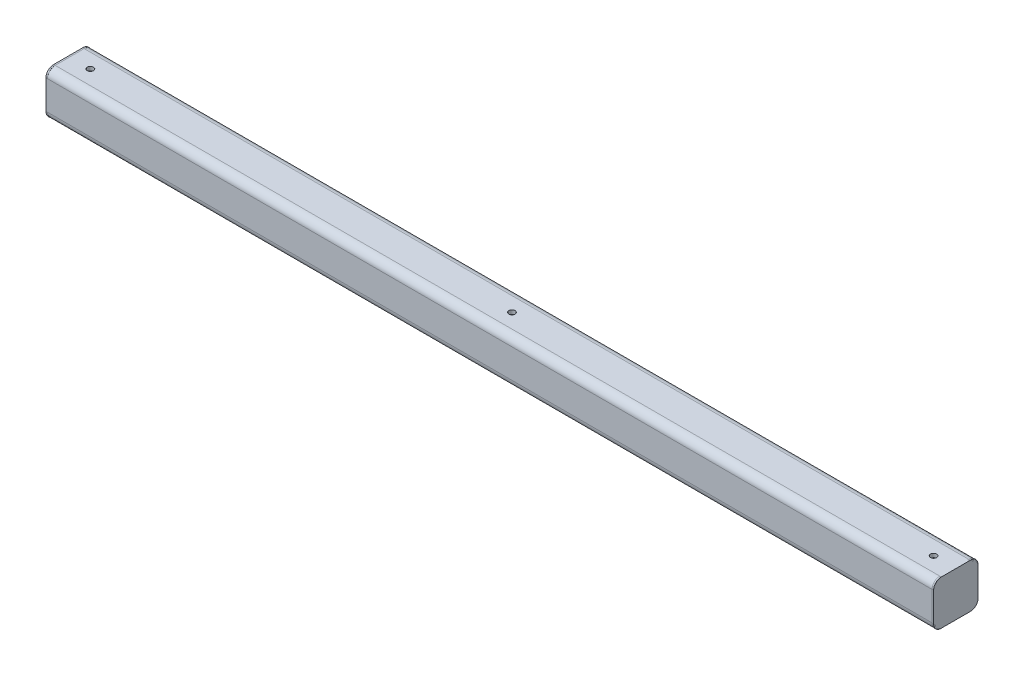
SolidWorks part; units mm, degrees
ref_plane "前视基准面" through (0, 0, 0) normal (0, 0, 1) x (1, 0, 0)
ref_plane "上视基准面" through (0, 0, 0) normal (0, 1, 0) x (1, 0, 0)
ref_plane "右视基准面" through (0, 0, 0) normal (1, 0, 0) x (0, 0, -1)
sketch3d "3D草图1"
  line L0 (0, 0, 0) -> (600, 0, 0)
  dimension "D1" = 600
other "结构构件1"
ref_plane "基准面1" through (0, 0, 0) normal (1, 0, 0) x (0, 0, -1)
sketch "Sketch1" plane through (0, 0, 0) normal (1, 0, 0) x (0, 0, -1)
  line L0 (-9.8, -12.4) -> (9.8, -12.4)
  line L1 (-12.4, -9.8) -> (-12.4, 9.8)
  line L2 (9.8, 12.4) -> (-9.8, 12.4)
  line L3 (12.4, 9.8) -> (12.4, -9.8)
  line L4 (-9.8, -15) -> (9.8, -15)
  line L5 (-15, -9.8) -> (-15, 9.8)
  line L6 (9.8, 15) -> (-9.8, 15)
  line L7 (15, 9.8) -> (15, -9.8)
  arc A0 (15, 9.8) -> (9.8, 15) centre (9.8, 9.8) ccw
  arc A1 (9.8, -15) -> (15, -9.8) centre (9.8, -9.8) ccw
  arc A2 (-15, -9.8) -> (-9.8, -15) centre (-9.8, -9.8) ccw
  arc A3 (-9.8, 15) -> (-15, 9.8) centre (-9.8, 9.8) ccw
  arc A4 (-9.8, 12.4) -> (-12.4, 9.8) centre (-9.8, 9.8) ccw
  arc A5 (12.4, 9.8) -> (9.8, 12.4) centre (9.8, 9.8) ccw
  arc A6 (9.8, -12.4) -> (12.4, -9.8) centre (9.8, -9.8) ccw
  arc A7 (-12.4, -9.8) -> (-9.8, -12.4) centre (-9.8, -9.8) ccw
  point P0 (-15, 0)
  point P1 (15, 0)
  point P2 (0, 15)
  point P3 (0, -15)
  point P4 (0, 0)
  point P5 (-15, -15)
  point P6 (15, -15)
  point P7 (15, 15)
  point P8 (-15, 15)
  point P33 (0, 0)
  dimension "D1" = 5.2
  dimension "Thickness" = 2.6
  dimension "V_leg" = 30
sketch "草图1" plane through (0, 0, 0) normal (-1, 0, 0) x (0, 0, 1)
  line L1 (10, 15) -> (-10, 15)
  line L2 (15, 10) -> (15, -10)
  line L3 (10, -15) -> (-10, -15)
  line L4 (-15, 10) -> (-15, -10)
  line L5 (15, 15) -> (-15, -15) construction
  line L6 (15, -15) -> (-15, 15) construction
  arc A0 (-10, -15) -> (-15, -10) centre (-10, -10) cw
  arc A1 (15, -10) -> (10, -15) centre (10, -10) cw
  arc A2 (10, 15) -> (15, 10) centre (10, 10) cw
  arc A3 (-10, 15) -> (-15, 10) centre (-10, 10) ccw
  point P0 (0, 0)
  dimension "D1" = 5
extrude "凸台-拉伸1" add sketch "草图1" against normal blind 1 separate body
sketch "草图2" plane through (600, 0, 0) normal (1, 0, 0) x (0, 0, -1)
  line L1 (10, 15) -> (-10, 15)
  line L2 (15, 10) -> (15, -10)
  line L3 (10, -15) -> (-10, -15)
  line L4 (-15, 10) -> (-15, -10)
  line L5 (15, 15) -> (-15, -15) construction
  line L6 (15, -15) -> (-15, 15) construction
  arc A0 (-10, -15) -> (-15, -10) centre (-10, -10) cw
  arc A1 (15, -10) -> (10, -15) centre (10, -10) cw
  arc A2 (10, 15) -> (15, 10) centre (10, 10) cw
  arc A3 (-10, 15) -> (-15, 10) centre (-10, 10) ccw
  point P0 (0, 0)
  dimension "D1" = 5
extrude "凸台-拉伸2" add sketch "草图2" against normal blind 1 separate body
hole_wizard "M5 螺纹孔1" positions "草图6" profile "草图5" tap size "M5" standard "Iso" end condition through all
sketch "草图6" plane through (0, -15, 0) normal (0, -1, 0) x (-1, 0, 0)
  point P0 (-15, 0)
  point P3 (-300, 0)
  point P6 (-585, 0)
sketch "草图5" plane through (15, -15, 0) normal (1, 0, 0) x (0, 0, -1)
  line L0 (0, 0) -> (0, 30)
  line L1 (0, 30) -> (2.1, 30)
  line L2 (2.1, 30) -> (2.1, 0)
  line L5 (2.1, 0) -> (0, 0)
  line L11 (0, -6.35) -> (0, 107.95) construction
  dimension "通孔螺纹孔钻头直径" = 4.2
  dimension "通孔螺纹孔钻头深度" = 30
cosmetic thread "孔螺蚊线1" parameters "D2"=5
cosmetic thread "孔螺蚊线2" parameters "D2"=5
cosmetic thread "孔螺蚊线3" parameters "D2"=5
